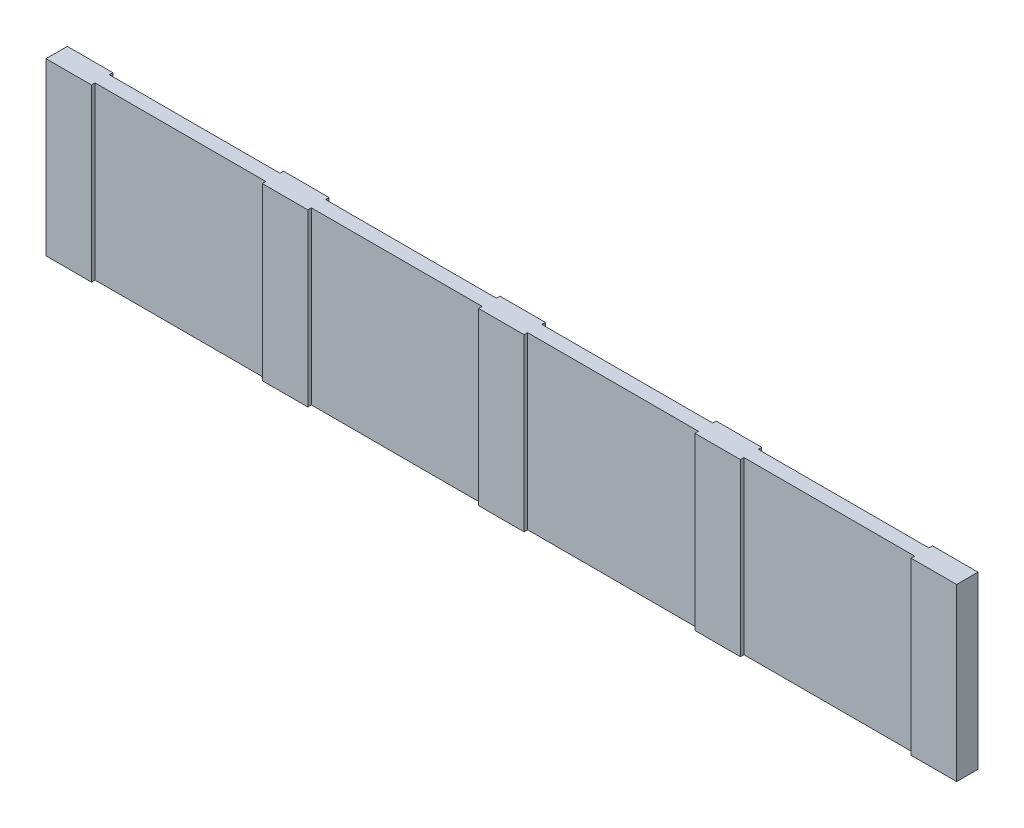
from build123d import *

# Parameters (mm, degrees)
SKETCH1_W           = 1270
SKETCH1_H           = 240
BOSS_EXTRUDE1_DEPTH = 20
SKETCH3_W           = 64
SKETCH3_H           = 30
BOSS_EXTRUDE2_DEPTH = 240


with BuildPart() as part:
    # Sketch1 → Boss-Extrude1 (new body)
    with BuildSketch(Plane.XY):
        with Locations((635, 120)):
            Rectangle(SKETCH1_W, SKETCH1_H)
    extrude(amount=BOSS_EXTRUDE1_DEPTH)

    # Sketch3 → Boss-Extrude2 (add)
    with BuildSketch(Plane.XZ):
        with Locations((32, 10)):
            Rectangle(SKETCH3_W, SKETCH3_H)
        with Locations((336, 10)):
            Rectangle(SKETCH3_W, SKETCH3_H)
        with Locations((640, 10)):
            Rectangle(SKETCH3_W, SKETCH3_H)
        with Locations((944, 10)):
            Rectangle(SKETCH3_W, SKETCH3_H)
        with Locations((1248, 10)):
            Rectangle(SKETCH3_W, SKETCH3_H)
    extrude(amount=-BOSS_EXTRUDE2_DEPTH)


solid = part.part
